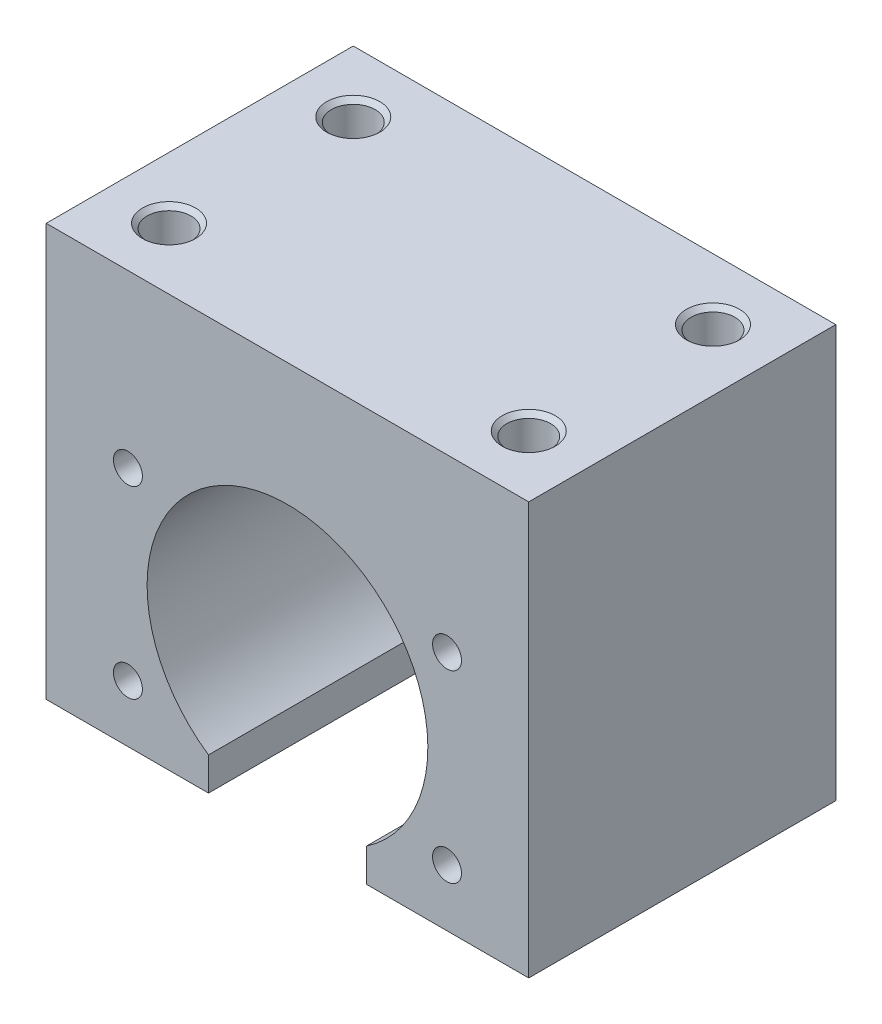
SolidWorks part; units mm, degrees
ref_plane "前视基准面" through (0, 0, 0) normal (0, 0, 1) x (1, 0, 0)
ref_plane "上视基准面" through (0, 0, 0) normal (0, 1, 0) x (1, 0, 0)
ref_plane "右视基准面" through (0, 0, 0) normal (1, 0, 0) x (0, 0, -1)
sketch "草图1" plane through (0, 0, 0) normal (0, 0, 1) x (1, 0, 0)
  line L0 (-27.5, 30) -> (27.5, 30)
  line L1 (27.5, 30) -> (27.5, -17)
  line L2 (27.5, -17) -> (9, -17)
  line L3 (9, -17) -> (9, -13.2288)
  line L4 (-27.5, 30) -> (-27.5, -17)
  line L5 (-27.5, -17) -> (-9, -17)
  line L6 (-9, -17) -> (-9, -13.2288)
  arc A0 (9, -13.2288) -> (-9, -13.2288) centre (0, 0) ccw
extrude "凸台-拉伸1" add sketch "草图1" along normal mid plane 35
hole_wizard "M4 螺纹孔1" positions "草图3" profile "草图2" tap size "M4" standard "GB"
sketch "草图3" plane through (0, 0, 17.5) normal (0, 0, 1) x (1, 0, 0)
  circle A0 centre (18.1865, 10.5) radius 2.25 construction
  circle A1 centre (18.1865, -10.5) radius 2.25 construction
  circle A2 centre (-18.1865, -10.5) radius 2.25 construction
  circle A3 centre (-18.1865, 10.5) radius 2.25 construction
  point P1 (18.1865, 10.5)
  point P5 (18.1865, -10.5)
  point P9 (-18.1865, -10.5)
  point P13 (-18.1865, 10.5)
cosmetic thread "孔螺蚊线1" parameters "D1"=6, "D2"=4
cosmetic thread "孔螺蚊线2" parameters "D1"=6, "D2"=4
cosmetic thread "孔螺蚊线3" parameters "D1"=6, "D2"=4
cosmetic thread "孔螺蚊线4" parameters "D1"=6, "D2"=4
sketch "草图2" plane through (18.1865, 10.5, 17.5) normal (1, 0, 0) x (0, -1, 0)
  line L0 (0, 0) -> (0, 10.4914)
  line L1 (0, 10.4914) -> (1.65, 9.5)
  line L2 (1.65, 9.5) -> (1.65, 0)
  line L5 (1.65, 0) -> (0, 0)
  line L10 (0, 10.4914) -> (-1.65, 9.5) construction
  line L11 (0, -6.35) -> (0, 107.95) construction
  dimension "螺纹孔钻头直径" = 3.3
  dimension "螺纹孔钻头深度" = 9.5
  dimension "导头角度" = 118
sketch "草图4" plane through (0, 30, 0) normal (0, 1, 0) x (1, 0, 0)
  line L0 (27.5, -17.5) -> (27.5, 17.5) construction
  line L1 (-20.5, -10.5) -> (20.5, -10.5)
  line L2 (-20.5, -10.5) -> (-20.5, 10.5)
  line L3 (-20.5, 10.5) -> (20.5, 10.5)
  line L4 (20.5, -10.5) -> (20.5, 10.5)
  line L5 (-20.5, -10.5) -> (20.5, 10.5) construction
  line L6 (-20.5, 10.5) -> (20.5, -10.5) construction
  line L7 (27.5, -17.5) -> (-27.5, -17.5) construction
  point P0 (0, 0)
  dimension "D1" = 7
  dimension "D2" = 7
hole_wizard "M6 螺纹孔1" positions "3D草图1" profile "草图5" tap size "M6" standard "GB"
sketch3d "3D草图1"
  point P0 (-20.5, 30, 10.5)
  point P3 (-20.5, 30, -10.5)
  point P6 (20.5, 30, -10.5)
  point P9 (20.5, 30, 10.5)
sketch "草图5" plane through (-20.5, 30, 10.5) normal (1, 0, 0) x (0, 0, 1)
  line L0 (0, 0) -> (0, 13.5022)
  line L1 (0, 13.5022) -> (2.5, 12)
  line L2 (2.5, 12) -> (2.5, 0.525)
  line L3 (2.5, 0.525) -> (3.025, 0)
  line L5 (3.025, 0) -> (0, 0)
  line L6 (-2.5, 0.525) -> (-3.025, 0) construction
  line L10 (0, 13.5022) -> (-2.5, 12) construction
  line L11 (0, -6.35) -> (0, 107.95) construction
  dimension "螺纹孔钻头直径" = 5
  dimension "螺纹孔钻头深度" = 12
  dimension "近端锥形沉头孔直径" = 6.05
  dimension "近端锥形沉头孔角度" = 90
  dimension "导头角度" = 118
cosmetic thread "孔螺蚊线5" parameters "D1"=8, "D2"=6
cosmetic thread "孔螺蚊线6" parameters "D1"=8, "D2"=6
cosmetic thread "孔螺蚊线7" parameters "D1"=8, "D2"=6
cosmetic thread "孔螺蚊线8" parameters "D1"=8, "D2"=6
equation "\"D3@草图1\"=\"D2@草图1\""
